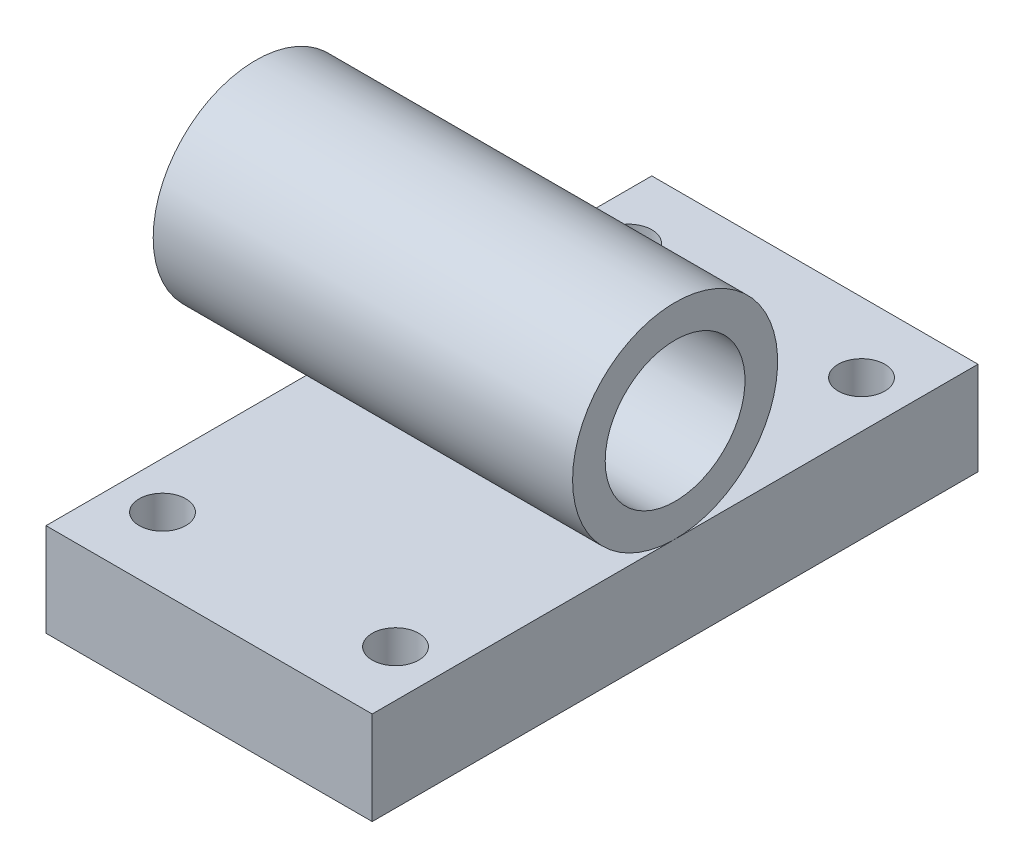
SolidWorks part; units mm, degrees
material "A3"
ref_plane "前视基准面" through (0, 0, 0) normal (0, 0, 1) x (1, 0, 0)
ref_plane "上视基准面" through (0, 0, 0) normal (0, 1, 0) x (1, 0, 0)
ref_plane "右视基准面" through (0, 0, 0) normal (1, 0, 0) x (0, 0, -1)
sketch "草图1" plane through (0, 0, 0) normal (0, 1, 0) x (1, 0, 0)
  line L0 (-25, -50) -> (25, -50) construction
  line L1 (-35, -65) -> (35, -65)
  line L2 (-35, -65) -> (-35, 65)
  line L3 (-35, 65) -> (35, 65)
  line L4 (35, -65) -> (35, 65)
  line L5 (-35, -65) -> (35, 65) construction
  line L6 (-35, 65) -> (35, -65) construction
  line L7 (-25, -50) -> (-25, 50) construction
  circle A0 centre (-25, -50) radius 5
  circle A1 centre (25, -50) radius 5
  circle A3 centre (25, 50) radius 5
  circle A5 centre (-25, 50) radius 5
  point P0 (0, 0)
  dimension "D3" = 10
  dimension "D5" = 50
  dimension "D1" = 130
  dimension "D2" = 70
  dimension "D4" = 10
  dimension "D8" = 50
  dimension "D9" = 100
  dimension "D6" = 2
  dimension "D7" = 2
extrude "凸台-拉伸1" add sketch "草图1" along normal blind 20
sketch "草图2" plane through (0, 0, 0) normal (0, 0, 1) x (1, 0, 0)
  line L0 (-55, 42) -> (76.0867, 42) construction
  line L1 (-35, 0) -> (35, 0) construction
  line L10 (-55, 50) -> (-47, 50)
  line L12 (-55, 50) -> (-55, 64)
  line L13 (-55, 64) -> (35, 64)
  line L14 (35, 64) -> (35, 57)
  line L15 (35, 57) -> (-47, 57)
  line L16 (-47, 57) -> (-47, 50)
  line L18 (35, 20) -> (35, 0) construction
  dimension "D1" = 42
  dimension "D2" = 44
  dimension "D3" = 90
  dimension "D4" = 8
  dimension "D5" = 16
  dimension "D6" = 30
revolve "旋转1" add sketch "草图2" angle 360 about L0
hole_wizard "M8 螺纹孔1" positions "草图3" profile "草图4" tap size "M8" standard "GB" end condition through all
sketch "草图3" plane through (0, 0, 0) normal (0, 0, 1) x (1, 0, 0)
  line L0 (35, 20) -> (35, 64) construction
  point P0 (15, 42)
  dimension "D1" = 20
  dimension "D2" = 42
sketch "草图4" plane through (15, 42, 0) normal (1, 0, 0) x (0, -1, 0)
  line L0 (0, 0) -> (0, 65)
  line L1 (0, 65) -> (3.4, 65)
  line L2 (3.4, 65) -> (3.4, 0)
  line L5 (3.4, 0) -> (0, 0)
  line L11 (0, -6.35) -> (0, 107.95) construction
  dimension "通孔螺纹孔钻头直径" = 6.8
  dimension "通孔螺纹孔钻头深度" = 65
cosmetic thread "孔螺蚊线1" parameters "D2"=8
